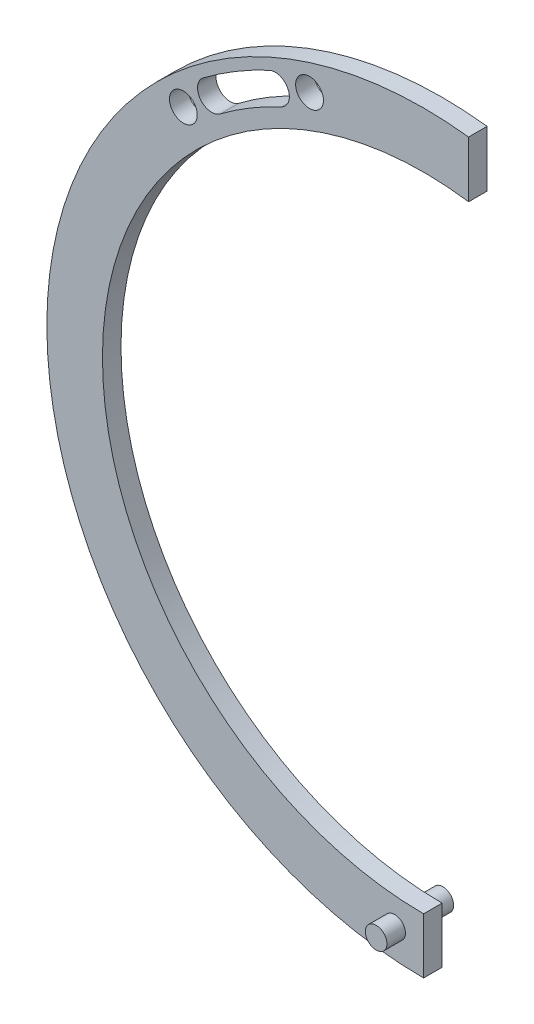
SolidWorks part; units mm, degrees
ref_plane "Front Plane" through (0, 0, 0) normal (0, 0, 1) x (1, 0, 0)
ref_plane "Top Plane" through (0, 0, 0) normal (0, 1, 0) x (1, 0, 0)
ref_plane "Right Plane" through (0, 0, 0) normal (1, 0, 0) x (0, 0, -1)
sketch "Sketch1" plane through (0, 0, 0) normal (0, 0, 1) x (1, 0, 0)
  line L0 (-267.317, 384.5719) -> (-267.3016, 354.3158)
  line L1 (-291.5852, 9.4358) -> (-291.5852, -20.5642)
  arc A1 (-267.317, 384.5719) -> (-291.5852, -20.5642) centre (-291.5852, 182.7307) ccw
  arc A2 (-291.5852, 9.4358) -> (-267.3016, 354.3158) centre (-291.5852, 182.7307) cw
extrude "Boss-Extrude1" add sketch "Sketch1" against normal up to surface (10 mm away)
sketch "Sketch2" plane through (0, 0, 0) normal (0, 0, 1) x (1, 0, 0)
  circle A0 centre (-307.2015, -4.5199) radius 5.8203
extrude "Boss-Extrude2" add sketch "Sketch2" along normal blind 10 and the other way blind 26 contours A0
sketch "Sketch7" plane through (0, 0, -10) normal (0, 0, -1) x (-1, 0, 0)
  circle A0 centre (421.224, 321.6328) radius 7.5
  circle A1 centre (353.1289, 362.4871) radius 7.5
  arc A2 (405.9195, 334.4794) -> (371.6835, 355.0219) centre (291.5852, 182.7307) ccw construction
  arc A3 (410.53, 340.5987) -> (374.9134, 361.9696) centre (291.5852, 182.7307) ccw
  arc A4 (401.309, 328.3602) -> (368.4535, 348.0743) centre (291.5852, 182.7307) ccw
  arc A5 (401.309, 328.3602) -> (410.53, 340.5987) centre (405.9195, 334.4794) ccw
  arc A6 (374.9134, 361.9696) -> (368.4535, 348.0743) centre (371.6835, 355.0219) ccw
  point P9 (389.3426, 345.6524)
  dimension "D1" = 190
extrude "Cut-Extrude4" cut sketch "Sketch7" against normal through all both and the other way through all
